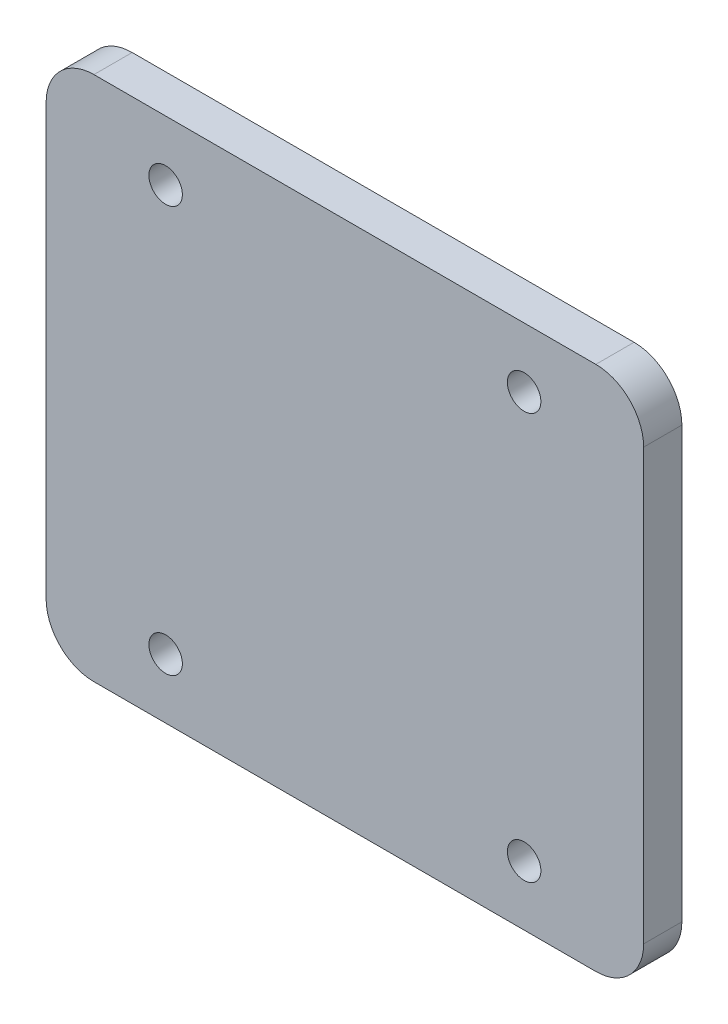
from build123d import *

# Parameters (mm, degrees)
SKETCH1_W           = 250
SKETCH1_H           = 220
BOSS_EXTRUDE1_DEPTH = 8
F_14_HOLE1_D        = 14
FILLET2_R           = 20


with BuildPart() as part:
    # Sketch1 → Boss-Extrude1 (new, symmetric)
    with BuildSketch(Plane.XY):
        Rectangle(SKETCH1_W, SKETCH1_H)
    extrude(amount=BOSS_EXTRUDE1_DEPTH, both=True)

    # Ø14 Hole1 (through all)
    with Locations(Plane.XY.offset(8)):
        with Locations((-75, 85), (75, 85), (75, -85), (-75, -85)):
            Hole(F_14_HOLE1_D / 2)

    # Fillet2
    fillet2_edges = [part.edges().sort_by_distance(p)[0] for p in [
        (-125, 110, 0),
        (125, 110, 0),
        (125, -110, 0),
        (-125, -110, 0),
    ]]
    fillet(fillet2_edges, radius=FILLET2_R)


solid = part.part
